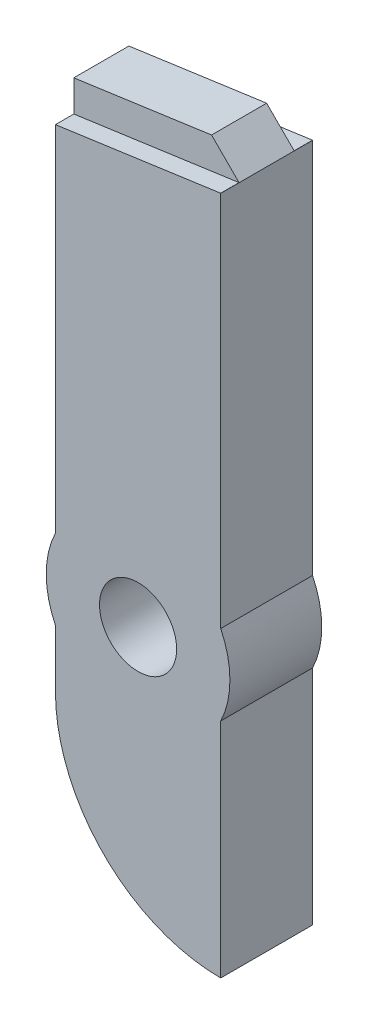
SolidWorks part; units mm, degrees
material "普通碳钢"
ref_plane "前视" through (0, 0, 0) normal (0, 0, 1) x (1, 0, 0)
ref_plane "上视" through (0, 0, 0) normal (0, 1, 0) x (1, 0, 0)
ref_plane "右视" through (0, 0, 0) normal (1, 0, 0) x (0, 0, -1)
sketch "草图1" plane through (0, 0, 0) normal (0, 0, 1) x (1, 0, 0)
  line L0 (-679.8242, 0) -> (730.2418, 0) construction
  line L1 (0, 451.3187) -> (0, -469.2088) construction
  line L2 (0, 0) -> (0, 121.2055)
  line L3 (0, 370) -> (-15, 385)
  line L4 (-15, 385) -> (-90, 374.4594)
  line L5 (-90, 374.4594) -> (-90, 164.7945)
  line L6 (0, 164.7945) -> (0, 370)
  line L7 (-90, 121.2055) -> (-90, 90)
  circle A1 centre (-45, 143) radius 21
  arc A2 (-90, 164.7945) -> (-90, 121.2055) centre (-45, 143) ccw
  arc A3 (0, 121.2055) -> (0, 164.7945) centre (-45, 143) ccw
  arc A4 (-90, 90) -> (0, 0) centre (0, 90) ccw
  dimension "D5" = 42
  dimension "D8" = 100
  dimension "D9" = 82
  dimension "D4" = 90
  dimension "D1" = 370
  dimension "D2" = 385
  dimension "D3" = 45
  dimension "D6" = 45
  dimension "D7" = 143
extrude "凸台-拉伸1" add sketch "草图1" along normal mid plane 50
ref_plane "基准面1" through (-36.6493, -5.1507, 0) normal (0.9903, 0.1392, 0) x (0, 0, -1)
sketch "草图2" plane through (-36.6493, -5.1507, 0) normal (0.9903, 0.1392, 0) x (0, 0, -1)
  line L0 (-15, 383.3408) -> (-15, 366.4408)
  line L1 (-25, 383.3408) -> (25, 383.3408) construction
  line L2 (-15, 366.4408) -> (-25, 366.4408)
  line L3 (-25, 163.1907) -> (-25, 366.3992) construction
  line L4 (-25, 366.4408) -> (-25, 383.3408)
  line L5 (-25, 383.3408) -> (-15, 383.3408)
  line L6 (15, 383.3408) -> (15, 366.4408)
  line L7 (15, 366.4408) -> (25, 366.4408)
  line L8 (25, 163.1907) -> (25, 366.3992) construction
  line L9 (25, 366.4408) -> (25, 383.3408)
  line L10 (25, 383.3408) -> (15, 383.3408)
  line L11 (0, 80.9) -> (0, -80.9) construction
  dimension "D1" = 16.9
  dimension "D2" = 16.9
  dimension "D3" = 15
  dimension "D4" = 15
extrude "切除-拉伸1" cut sketch "草图2" along normal through all both and the other way through all
